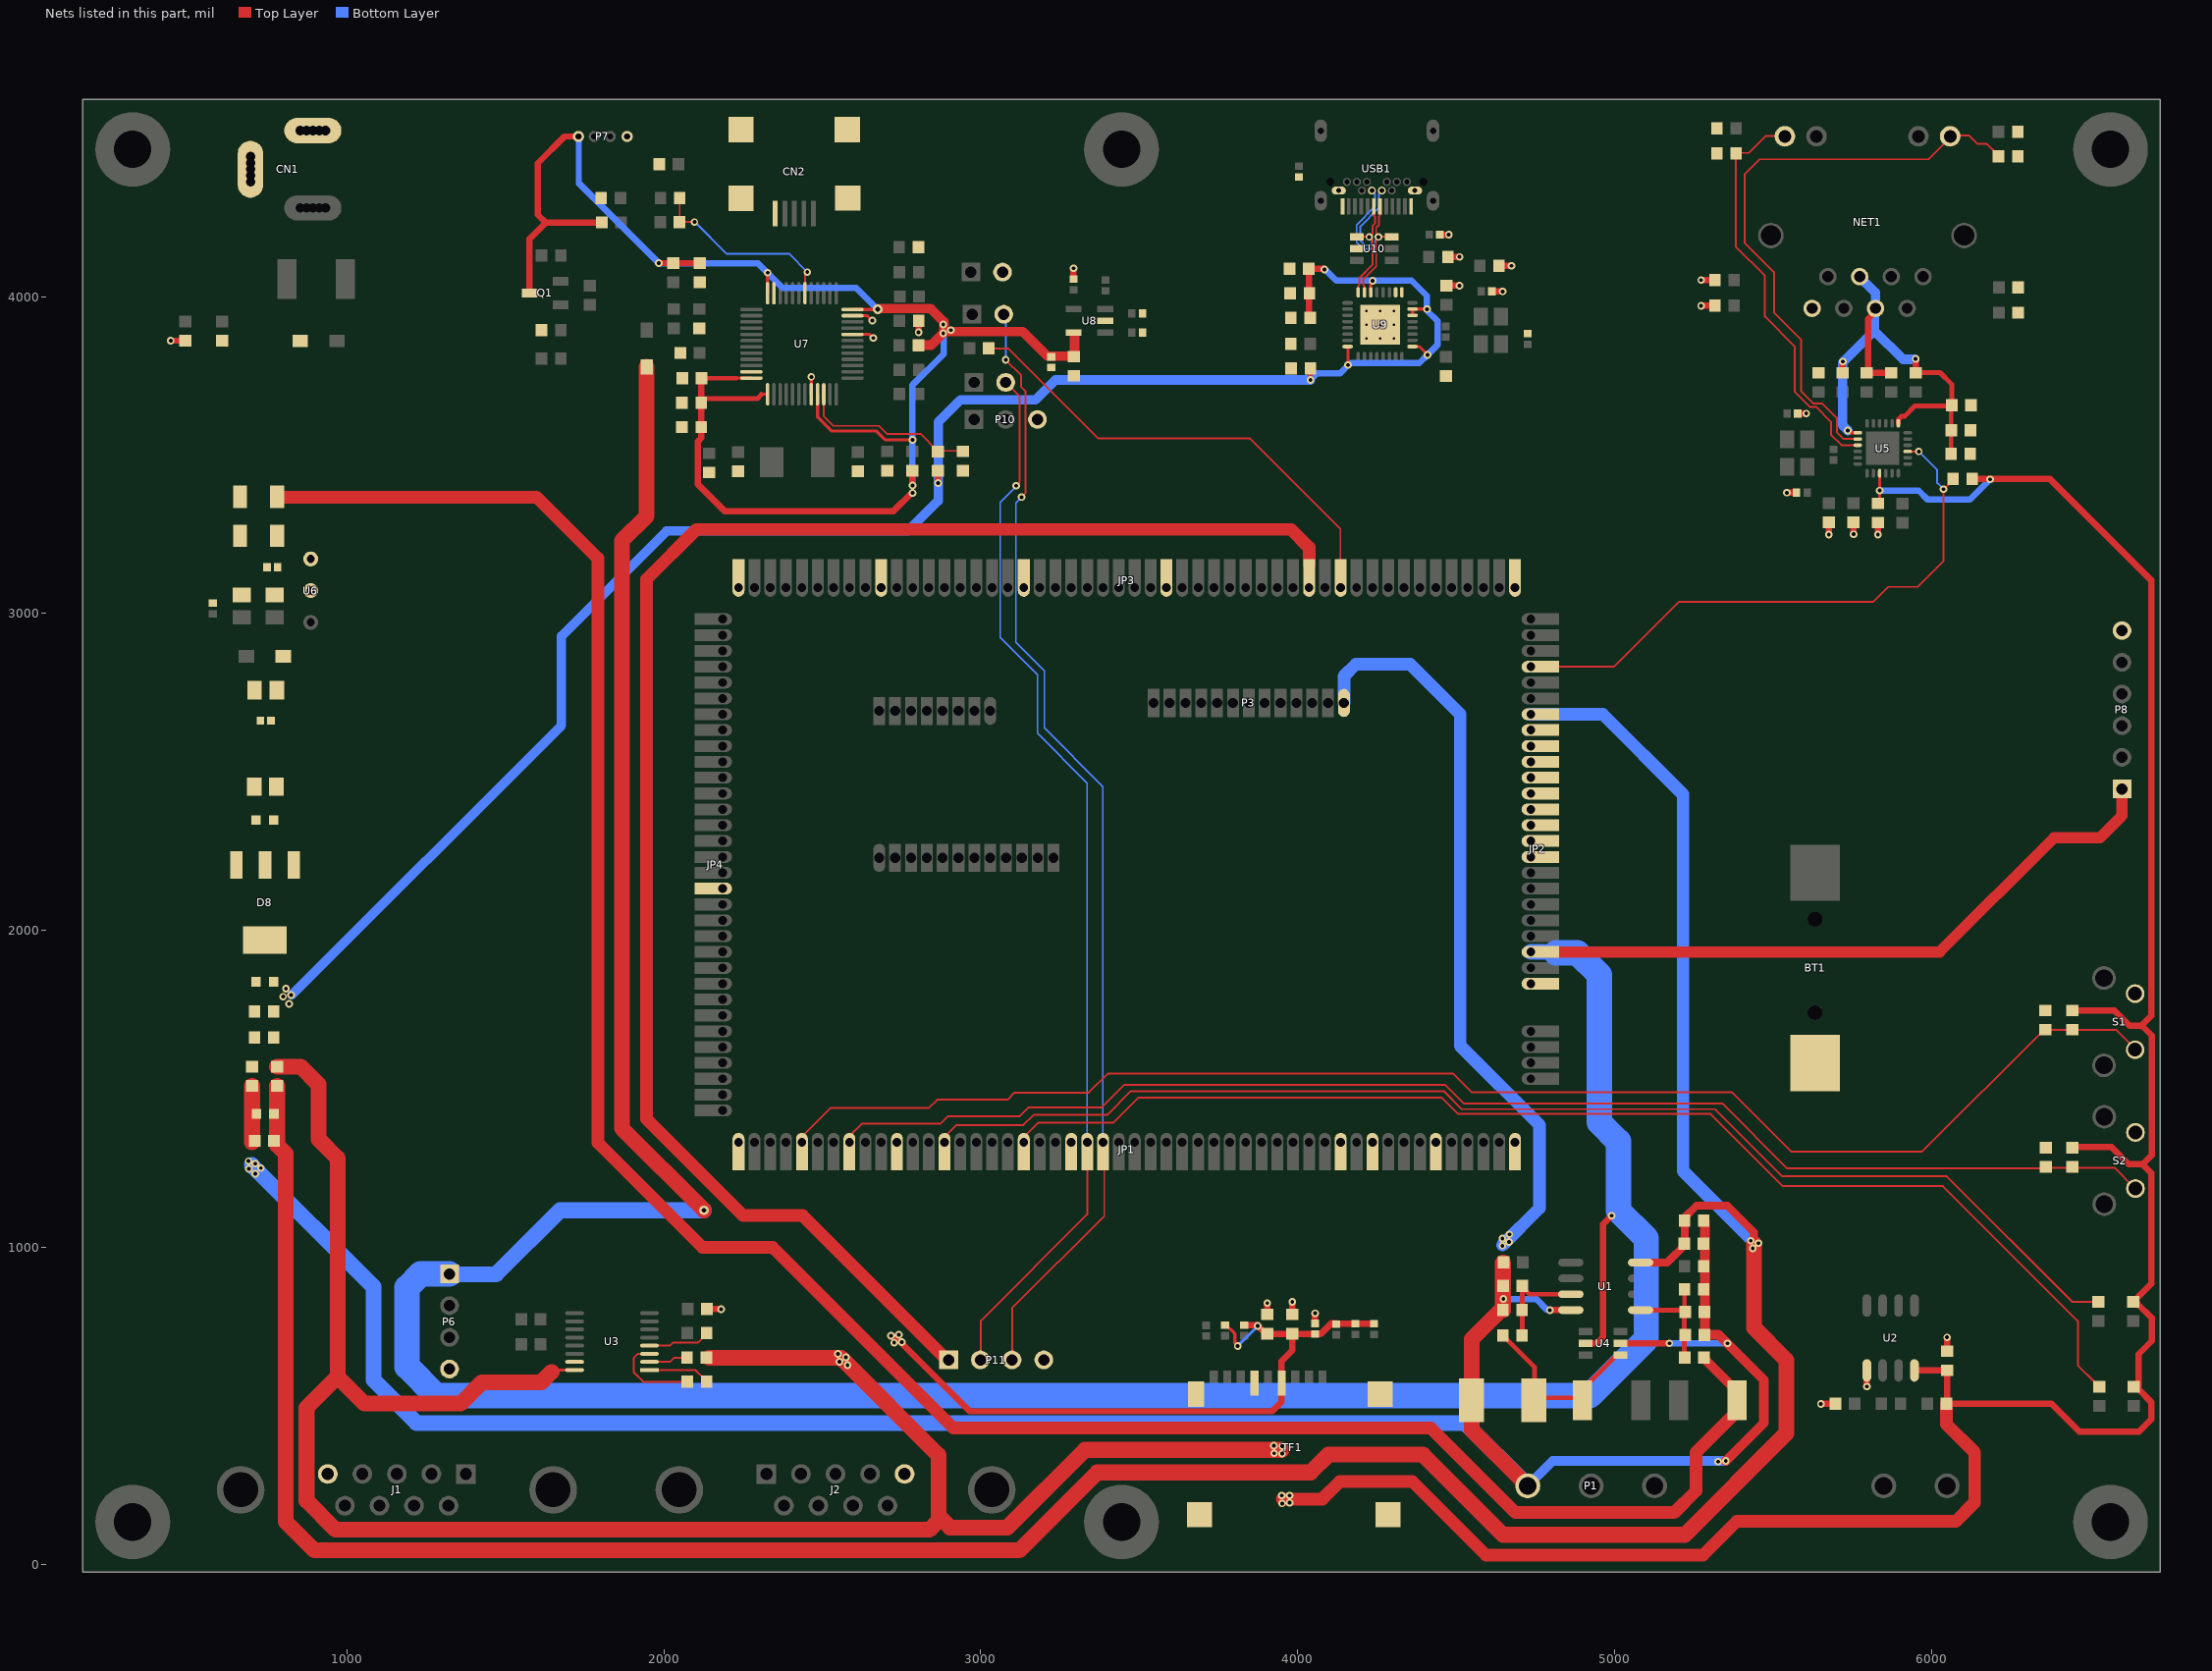
[diagram p0: the nets of this part, all layers, seen from the top]
# Altium PCB MISC105202-15.PcbDoc (part 2 of 4)
Units mil, origin at the board's own origin, x right, y up, seen from the top; angles counter-clockwise.
Board outline 6555.12 x 4645.67 mil, 2 copper layers (Top Layer, Bottom Layer); 182 components, 258 nets, 994 pads, 145 vias.
Unrouted connection lines stored in the file: 1.

## Footprints (in the part's own frame and the unit in brackets; to place one, negate y for a bottom-side part, rotate by r counter-clockwise, add the part's x,y. Pads: shape width x height; smd on the part's side, far side on the other; paste and mask are expansions set on the pad) (continued)
SMD-3225_4P [mm]
  rect 1.4x1.15 smd: 1(-1.1,-0.8) 2(1.1,-0.8) 3(1.1,0.8) 4(-1.1,0.8)
  silkscreen extent -2.1,-2.35 2.1,1.7, body extent -1.6,-1.25 1.6,1.25, height 0.61
SMD-5032_2P [mm]
  rect 1.9x2.4 smd: 1(-2.05,0) 2(2.05,0)
  silkscreen extent -3.32,-1.6 3.32,1.6
SO-8 [mil]
  oval 80x24 smd: 1(0,0) 2(0,-50) 3(0,-100) 4(0,-150) 5(220,-150) 6(220,-100) 7(220,-50) 8(220,0)
  silkscreen extent 60,-175 160,25
SOD-123 [mm]
  rect 1.25x1 smd: 1(1.475,0) 2(-1.475,0)
  silkscreen extent -0.5,-0.7 0.5,0.7, body extent -1.85,-0.77 1.85,0.78, height 1.35
SOIC-8_150mil [mm]
  oval 0.7x1.8 smd: 1(-1.905,-2.6) 2(-0.635,-2.6) 3(0.635,-2.6) 4(1.905,-2.6) 5(1.905,2.6) 6(0.635,2.6) 7(-0.635,2.6) 8(-1.905,2.6)
  silkscreen extent -2.9,-3.05 2.4,1.4
SOT23-5 [mil]
  rect 20x50 smd: 1(74.8,100) 2(37.4,100) 3(0,100) 4(0,0) 5(74.8,0)
  silkscreen extent 30,-5 45,-5
SOT-23(SOT-23-3) [mm]
  rect 1.25x0.7 smd: 1(1.25,-0.95) 2(1.25,0.95) 3(-1.25,0)
  silkscreen extent -0.65,-1.46 0.9,1.46, body extent -1.5,-1.5 1.5,1.5, height 1.3
SOT-23-6 [mm]
  rect 1.1x0.6 smd: 1(1.4,-0.95) 2(1.4,0) 3(1.4,0.95) 4(-1.4,0.95) 5(-1.4,0) 6(-1.4,-0.95)
  silkscreen extent -0.5,-1.87 1.73,1.4
SOT-223 [mm]
  rect 2.2x1 smd: 1(3,-2.3) 2(3,0) 3(3,2.3)
  rect 2.2x3.5 smd: 2(-3,0)
  silkscreen extent -1.4,-3 1.4,3, body extent -3.49,-3.24 3.49,3.24, height 1.64
TSSOP-16 [mm]
  rect 1.5x0.3 smd: 1(0,0)
  oval 1.5x0.3 smd: 2(0,-0.65) 3(0,-1.3) 4(0,-1.95) 5(0,-2.6) 6(0,-3.25) 7(0,-3.9) 8(0,-4.55) 9(6,-4.55) 10(6,-3.9) 11(6,-3.25) 12(6,-2.6) 13(6,-1.95) 14(6,-1.3) 15(6,-0.65) 16(6,0)
  silkscreen extent 1.58,-5.08 4.42,0.33
USB_TYPEC [mm]
  oval 1x1.8 hole 0.5 slot 1.3 at 90 deg: 0(-4.5,-2.805) 0(4.5,-2.805)
  oval 1x1.6 hole 0.5 slot 1.1 at 90 deg: 0(-4.5,2.805) 0(4.5,2.805)
  oval 0.64x0 hole 0.64 slot 0.95 at 0 deg unplated: 0(-3.725,1.295) 0(3.725,1.295)
  rect 0.3x1.3 smd: A1(-2.75,3.243) A2(-2.25,3.243) A3(-1.75,3.243) A4(-1.25,3.243) A5(-0.75,3.243) A6(-0.25,3.243) A7(0.25,3.243) A8(0.75,3.243) A9(1.25,3.243) A10(1.75,3.243) A11(2.25,3.243) A12(2.75,3.243)
  oval 1.14x0.64 hole 0.4 slot 0.9 at 0 deg: B1(3.05,1.995) B12(-3.05,1.995)
  round 0.65 hole 0.4: B2(2.4,1.295) B3(1.6,1.295) B4(1.2,1.995) B8(-0.8,1.295) B10(-1.6,1.295) B11(-2.4,1.295)
  round 0.64 hole 0.4: B5(0.8,1.295) B6(0.4,1.995) B7(-0.4,1.995) B9(-1.2,1.995)
  silkscreen extent -4.5,-6.46 4.5,3.96
ZY78xxLS-1000 [mm]
  round 1.2 hole 0.65: 1(-2.54,0) 2(0,0) 3(2.54,0)
  silkscreen extent -6,0.69 6,18.2

## Part data
BT1: library part Battery, "Multicell Battery"
C1 C2 C5 C6: library part "0603 100pF (101) 5% 50V", "贴片电容"
C3 C12 C25: library part "0603 10uF (106) 10% 10V", "贴片电容"
C4 C10 C22 C23 C24 C26 C58 C59 C60 C61 C62 C65 C66 C67: library part "0603 100nF (104) 10% 50V", "贴片电容"
C7 C8 C9 C11: library part CAP
C13 C14 C40 C41 C43: library part "0603 22uF (226) 20% 6.3V", "贴片电容"
C15 C30 C33 C35: library part "0402 100nF (104) 10% 16V", "贴片电容"
C16: library part "0603 22nF (223) 10% 50V", "贴片电容"
C17 C18 C20 C21: library part "0603 10pF (100) 5% 50V", "贴片电容"
C19 C28: library part "0402 10nF (103) 10% 50V", "贴片电容"
C27 C29 C54 C55 C57: library part "Cap Semi", "Capacitor (Semiconductor SIM Model)"
C31 C32 C34 C38: library part "0805 22uF (226) 20% 25V", "贴片电容"
C36 C37: library part "1206 10uF (106) 10% 50V", "贴片电容"
C39 C42 C44: library part CAP, "Capacitor"
C46 C47 C48 C49 C50 C51 C52: library part Capacitor_ST, "Capacitor 0402 / 0603 / 0805"
C53: library part "Cap Pol1", "Polarized Capacitor (Radial)"
C56: library part "0402 10uF (106) 20% 6.3V", "贴片电容"
C63 C64: library part "0402 20pF (200) 5% 50V", "贴片电容"
CN1: library part PJ202A
CN2: library part Mini-USB-AB
D3: library part "D Tunnel2", "Tunnel Diode - Dependent Source Model"
D4 D14: library part "0603 绿灯", "发光二极管"
D5 D9 D13: library part "0603 红灯", "发光二极管"
D6 D7 D12: library part "SOD-123 B5819W  SL", "肖特基二极管"
D8: library part CL1117-33
F1 F2 F3: library part "Fuse 2", "Fuse"
J1 J2: library part "D Connector 9", "Receptacle Assembly, 9 Position, Right Angle"
JP1 JP3: "Header, 50-Pin"
JP5 JP6: library part JP2
L1 L2: library part "0603 4.7uH 10%", "贴片电感"
P1 P10: library part "Header 3", "Header, 3-Pin"
P2 P9: library part "Header 2", "Header, 2-Pin"
P3: "Header, 13-Pin"
P4: "Header, 12-Pin"
P5: "Header, 8-Pin"
P6 P7 P11: library part "Header 4", "Header, 4-Pin"
P8: library part "Header 6", "Header, 6-Pin"
Q1: library part "SOT-23 SS8050 Y1", "三极管"
R1 R2 R3 R4 R28 R30 R31 R52: library part "0603 10KΩ (1002) 1%", "贴片电阻"
R5 R7: library part "0603 360Ω (3600) 1%", "贴片电阻"
R6: library part "0603 120Ω (1200) 1%", "贴片电阻"
R8 R9: library part "0603 100Ω (1000) 1%", "贴片电阻"
R11 R12 R13 R14 R15: library part "0402 47KΩ (4702) 1%", "贴片电阻"
R16: library part "0402 100Ω (1000) 1%", "贴片电阻"
R17 R19 R32 R57 R58 R59: library part Reszte, "Resistor"
R18 R20: library part "0603 680Ω (6800) 1%", "贴片电阻"
R21 R22 R23 R24: library part "0603 49.9Ω (49R9) 1%", "贴片电阻"
R25 R26 R29 R50 R51: library part "0603 510Ω (5100) 1%", "贴片电阻"
R27 R61: library part "0603 12KΩ (1202) 1%", "贴片电阻"
R33: library part RES-S
R34 R35 R48 R49 R54 R56: library part Res1, "Resistor"
R36 R37 R38 R39 R40 R41 R42 R43 R44 R45 R46 R47 R53 R55: library part Resistor_ST, "Resistor 0402 / 0603 / 0805"
R60: library part "0402 1MΩ (1004) 1%", "贴片电阻"
S1 S2: library part SW-PB
U1: library part OPA2335
U2: library part SP3485EN-L/TR_[C8963], "RS-485/RS-422"
U3: "RS232"
U4: library part SRV05-4-P-T7_[C85364], "TVS"
U5: library part LAN8742A-CZ-TR, "LAN8742A-CZ-TR - Small Footprint RMII 10/100 Ethernet, Transceiver with HP Auto-MDIX and flexPWR Technology SQFN-24"
U6: library part ZY78xxLS
U7: "Medium-density performance line ARM-based 32-bit MCU with 64KB Flash"
U8: library part TPS76901HDB
U9: library part USBD3300
U10: library part TPD4E001
USB1: library part USB_Type_C_Receptacle
Y1 Y3: library part "SMD-3225_4P  25MHZ 12PF 10PPM", "贴片晶振"
Y2: library part "SMD-5032_2P 8MHz 20ppm 20pF", "贴片晶振"

## Free pads (board coordinates)
  round 236.22 hole 118.11: 0(324.48,133.48) 0(324.48,4464.19) 0(3444.56,133.48) 0(3444.56,4464.19) 0(6564.64,133.48) 0(6564.64,4464.19)

## Via types
v1: diameter 24, hole 12, Top Layer to Bottom Layer, 128 vias
v2: diameter 19.68, hole 7.87, Top Layer to Bottom Layer, 9 vias
v3: diameter 50, hole 50, Top Layer to Bottom Layer, 4 vias
v4: diameter 30, hole 15, Top Layer to Bottom Layer, 2 vias
v5: diameter 137.8, hole 137.8, Top Layer to Bottom Layer, 2 vias

## Nets (pads, with @x,y where several pads share a name; then routed paths per layer and width w, separated by ;. In a path a pad name is that pad's centre, name@x,y a point inside that pad or via, vN(x,y) a via of type N, cw(c..) or ccw(c..) an arc to the next point about the centre after c; other vN are vias at no path point)
3V3: C8.1 C10.2 C13.2 C14.2 C15.2 C22.2 C40.2 C41.2 C42.2 C59.2 C60.2 C61.2 C62.2 D4.A D5.A D8.2 L1.1 R5.1 R11.2 R12.2 R13.2 R14.2 R15.2 R17.2 R19.2 R28.1 R43.1 TF1.4 U2.8 U3.16 U5.9 U9.6 U9.16 U9.25 U9.30 U9.31 | length 22661.3
  Top Layer w10: 1636,601 1648,613 U3.16@1718.78,613 ; R13.2@3771,754.73 3774.87,754.73 3802,727.6 3802,698 v1(3811,689) ; U9.16@4157.64,3842.1 4159,3840.74 v1(4159,3784) ; U9.6@4230.47,4013.36 4230.47,4043.47 v1(4237,4050) ; U9.25@4362.36,3842.1 4383.9,3842.1 v1(4410,3816) ; U9.30@4363,3943 4362.36,3943.64 U9.31@4362.36,3960.21 v1(4408.21,3960.21) ; C22.2@5836.16,3359.16 v1@5836.16,3393 ; v1(5836.16,3387.84) v1@5836.16,3393 ; U5.9@5836.16,3442.26 v1@5836.16,3393
  Top Layer w15: v1(4040.31,3736.69) C62.2@4040.31,3773
  Top Layer w20: C8.1@2134.31,652 C8.1@2144,652 ; v1@2716.5,718.5 2729.5,718.5 2965.44,482.56 3919.56,482.56 3949.69,512.69 TF1.4@3949.69,571.56 3949.69,641.69 3983,675 C13.2@3983,716 ; v1(2865.43,3411.57) R43.1@2865.43,3450.31 ; 2871,142 2874,145 ; R12.2@3831,754.73 3872.27,754.73 C14.2@3896,731 ; C14.2@3904,727.68 3904.69,727 4054,727 C15.2@4055,726 ; C61.2@4035,3931 4035.31,3931.31 C59.2@4035.31,4088 4082,4088 v1@4083,4087 ; C15.2@4059,726 4072,726 4106,760 4122,760 4123.27,758.73 R14.2@4182,758.73 R11.2@4241,758.73 ; U2.8@5946,611.64 6047.36,611.64 6049,610 6049,519 R5.1@6053,515 ; R5.1@6047.31,506 6379,506 6466,419 6655,419 6693,457 6693,512 6653,552 6653,663 6695,705 6695,777 D4.A@6649,823 ; R28.1@6128.31,3424 6374,3424 6693,3105 6693,1730 6662,1699 ; R17.2@6454,1747 6577,1747 6625,1699 6662,1699 ; R19.2@6455,1316 6568,1316 6622,1262 6666,1262 ; D4.A@6636,827.87 6693,884.87 6693,1235 6666,1262 ; D4.A@6644,826 D4.A@6649,826 ; 6661,1698 6662,1699 ; 6662,1699 6664,1699 6695,1668 6695,1291 6666,1262
  Top Layer w40: v1@3951,206 4078,206 4133,261 4362,261 4594,29 5279,29 5386,136 6077,136 6136,195 6136,353 6047.31,441.69 R5.1@6047.31,506
  Top Layer w50: L1.1@780,1570.31 854.69,1570.31 911,1514 911,1341 971,1281 971,592 ; 1646,607 1613,574 1426,574 1359,507 1056,507 971,592 ; C8.1@2144,652 2559,652 2867,344 2867,138 2838,109 965,109 873,201 873,494 971,592 ; 2874,145 2903,116 3084,116 3329,361 3949,361
  Bottom Layer w10: v1(3811,689) v1(3874,752)
  Bottom Layer w20: v1@4040,3736 4061,3757 4133,3757 4166,3790 4384,3790 v1(4410,3816) 4441,3847 4441,3923 4408,3956 4408,4002 4360,4050 v1(4237,4050) 4122,4050 v1@4087,4085 ; v1(4085,4085) v1@4086,4084 ; v1(5836.16,3387.84) 5959.16,3387.84 5988,3359 6121,3359 v1(6185,3423)
  Bottom Layer w30: v1@826.5,1796.5 1677,2647 1677,2928 2009,3260 2770,3260 2866,3356 2866,3604 2936,3674 3173,3674 3235.69,3736.69 v1(4040.31,3736.69)
  other v1: 3951,192 3975,194 3950,217 3975,217 3951,349 3926,350 3952,373 3925,374 2580,628 2554,639 2575,653 2550,664 2727,699 2751,701 2717,721 2742,724 818,1768 799,1791 824,1796 808,1816
3V3_E: C16.1 C23.2 C24.2 NET1.4 NET1.5 R21.2 R22.2 R23.2 R24.2 U5.1 U5.19 | length 1630.2
  Top Layer w10: v1(5736,3577) 5742.79,3570.21 U5.1@5767.26,3570.21
  Top Layer w15: U5.19@5895.21,3599.74 5895.21,3612.21 5905,3622 5915,3622 5948,3655 C16.1@6061,3655 ; R23.2@5962,3760 6027,3760 6063.68,3723.31 C16.1@6063.68,3657 ; C23.2@6061.68,3503 C16.1@6061.68,3650.69
  Top Layer w20: R22.2@5720,3759.32 v1(5720,3795) ; NET1.4@5825,3955 5799.68,3929.68 5799.68,3759.32 R24.2@5873,3759.32 ; R23.2@5950,3759.32 v1(5950,3803)
  Bottom Layer w30: v1(5736,3577) 5719,3594 5719,3791 5820,3892 ; NET1.5@5773.2,4062.63 5823,4012.83 NET1.4@5823,3971 ; NET1.4@5820,3962 5820,3892 ; v1@5947,3802 5910,3802 5820,3892
+3V3: JP3.37 P11.1 | length 5210.4
  Top Layer w30: JP3.37@4036,3147 JP3.37@4036,3155
  Top Layer w40: P11.1@2899,645 2893,645 2438,1100 2251,1100 1946,1405 1946,3108 2103,3265 3979,3265 4036,3208 JP3.37@4036,3155
+3V3_ST_LINK: C46.2 C47.2 C48.2 C49.2 C55.2 C56.2 D14.A P7.1 Q1.3 R38.1 R41.2 R49.1 U7.1 U7.9 U7.24 U7.36 U7.48 U8.5 | length 5585.1
  Top Layer w10: 2230,3742.73 U7.48@2276.55,3742.73 ; 2307.45,3691.55 U7.1@2327.73,3691.55 ; U7.36@2327.73,4010.45 v1(2327.73,4075.27) ; U7.9@2485.21,3691.55 2485.21,3619.79 2529,3576 2670,3576 2698,3548 v1(2785,3548) ; U7.24@2595.45,3959.27 2645.73,3959.27 2646,3959
  Top Layer w12: 2646,3959 v4@2677,3959
  Top Layer w15: C48.2@2119.31,3733.31 C48.2@2119.31,3742 2230,3742 ; C49.2@2132,3678 2296,3678 2307.45,3689.45 2307.45,3691.55
  Top Layer w20: Q1.3@1576.79,4011 1576.79,4181.79 1628,4233 ; P7.1@1728,4505 1687,4505 1603,4421 1603,4258 1628,4233 ; D14.A@1804,4235 1802,4233 1628,4233 ; v1(1984.31,4105.31) R38.1@2030,4105.31 ; R38.1@2035,4108 2037.69,4105.31 C46.2@2114,4105.31 ; C48.2@2122,3736 2119.31,3733.31 2118,3732 2118,3656 2118.31,3655.69 C47.2@2118.31,3588 2118.31,3553.31 2108,3543 2108,3407 2192,3323 2725,3323 v1@2783.5,3381.5 ; v1(2785,3404) R41.2@2785,3450.68
  Top Layer w30: v4@2677,3961 2677.71,3961.71 2842.29,3961.71 2884,3920 2884,3887 2844,3847 R49.1@2810,3847 ; v1@2886,3889 3133,3889 3210,3812 3291,3812 3296,3817 U8.5@3296,3880
  Bottom Layer w20: P7.1@1732,4502 1732,4357.63 v1(1984.31,4105.31) 1983,4104 2298,4104 2311,4091 ; v1@2325,4077 2311,4091 ; v4(2675,3960) 2674,3960 2607,4027 2375,4027 2311,4091 ; v1(2785,3404) v1(2785,3548) 2785,3721 2884,3820 v1@2884,3882
  other v1: 2785,3380 2882,3884 2906,3894 2882,3912
+5V: C34.2 C35.1 C38.2 C39.2 D7.2 D8.1 D12.1 JP2.11 P6.1 P8.1 U4.5 | length 12105.7
  Top Layer w20: U4.5@4907.88,697 4944,697 4964,717 4964,1073 v1(4991,1100)
  Top Layer w35: JP2.11@4780.49,1931.87 6025.87,1931.87 6386,2292 6531,2292 6601,2362 P8.1@6601,2436
  Top Layer w50: D12.1@1946,3777.93 1946,3307 1868,3229 1868,1376 v4(2127,1117)
  Bottom Layer w50: P6.1@1317,915 1471,915 1673,1117 v4(2127,1117) ; JP2.11@4736,1931.87 4811.87,1931.87 4816,1936
  Bottom Layer w80: P6.1@1324,916 1233,916 1190,873 1190,624 1282,532 4922,532 5100,710 5100,760 5100,1028 5012,1116 5012,1334 4952,1394 4952,1860 4883,1929 4816,1929
A3V3: C3.2 C4.2 C43.2 C44.2 JP2.26 L1.2 U1.8 | length 9790.7
  Top Layer w25: U1.8@5082,952 5166,952 5221,1007 5221,1094 5258,1131 5356,1131 5439,1048 v1@5439,1027
  Top Layer w50: L1.2@780,1509.68 780,1323 807,1296 807,135 898,44 3122,44 3368,290 4041,290 4097,346 4395,346 4648,93 5222,93 5542,413 5542,644 5440,746 5440,1012
  Bottom Layer w40: JP2.26@4736,2681.87 4963.13,2681.87 5216,2429 5216,1241 5441,1016
  other v1: 5436,997 5454,1013 5430,1021
AGND: C1.1 C2.1 C3.1 C4.1 C5.1 C6.1 C12.1 C43.1 C44.1 D3.1 L2.2 P1.3 P3.1 R2.1 R4.1 U1.4 U4.2 | length 10084.7
  Top Layer w20: v1(4796,802) U1.4@4862,802 ; U4.2@5018.12,697 v1(5173,697)
  Top Layer w30: C4.1@5282,1086 5285,1083 5285,940 5285,725.68 C12.1@5283.31,724 5328,724 5471,581 5471,446 v1(5351,326)
  Top Layer w50: C43.1@701,1331 701,1336 L2.2@701,1509.68 ; R2.1@4643,804 4549,710 D3.1@4549,518 4549,424 P1.3@4717,256 ; R2.1@4647.69,802 4647.69,950.69 C1.1@4648,951
  Bottom Layer w20: v1(4649,837) 4753,837 4788,802 v1(4796,802) ; v1(5173,697) v1(5356,697)
  Bottom Layer w30: P1.3@4737,258 4805,326 v1(5351,326)
  Bottom Layer w40: P3.1@4146,2717.62 4146,2802 4184,2840 4355,2840 4513,2682 4513,1636 4763,1386 4763,1124 v1@4646,1007
  Bottom Layer w50: v1@700,1260 1084,876 1084,582 1220,446 4527.37,446 P1.3@4726,247.37
  other v1: 5327,324 4646,1005 4667,1017 4646,1028 4668,1041 711,1232 691,1248 729,1250 711,1264 690,1272
AIN1: D3.2 F1.2 R1.2 U4.1 | length 560.6
  Top Layer w15: R1.2@4647.68,722 4748,621.68 D3.2@4748,559 ; D3.2@4761,523 4763,525 F1.2@4898,525 ; F1.2@4898,518 F1.2@4898,525 ; F1.2@4918,543 4900,525 F1.2@4898,525 ; U4.1@5011,659 5006,659 4898,551 F1.2@4898,525
AIN2: C30.1 C36.2 C37.2 D6.2 F3.2 R3.2 R33.1 U6.1 | length 7419.2
  Top Layer w30: R3.2@5287,645 5387,545 F3.2@5387,518 F3.2@5387,483
  Top Layer w40: C36.2@782,3367 1599,3367 1792,3174 1792,1330 2122,1000 2344,1000 2914,430 4420,430 4687,163 5188,163 5257,232 5257,353 F3.2@5387,483
AIN_1: R43.2 R44.2 U7.10 | length 549.7
  Top Layer w6: U7.10@2504.9,3691.55 2504.9,3622.1 2535,3592 2679,3592 2704,3567 2810,3567 2864,3513 R44.2@2940,3513
ARM_NRST: JP3.39 R36.2 | length 1477.4
  Top Layer w6: R36.2@3025.32,3836 3087,3836 3371,3552 3440,3552 3850,3552 4135,3267 JP3.39@4135,3135
ARM_SWO: R37.2
ARM_TCK: JP1.23 JP5.2 P11.2 | length 3318.1
  Top Layer w6: P11.2@3001,661 3001,769 3336,1104 JP1.23@3336,1287.38 ; JP5.2@3079,3729 3123,3685 3123,3414 v1(3112,3403)
  Bottom Layer w4: 3061.3,3230.7 3061.3,3229 ; v1@3111,3400 3061.3,3350.3 3061.3,3229 ; JP1.23@3336,1331.87 3336,2465 3179,2622 3179,2807 3061.3,2924.7 3061.3,3229
ARM_TMS: JP1.24 JP6.2 P11.3 | length 3539.5
  Top Layer w6: v1(3079,3800) 3128,3751 3128,3715 3142,3701 3142,3380 v1(3129,3367) ; P11.3@3099,645 3099,808 3390,1099 JP1.24@3390,1317
  Bottom Layer w4: v1(3129,3367) 3111,3349 3111,2909 3201,2819 3201,2639 3386,2454 3386,1380 JP1.24@3386,1331.87
  Bottom Layer w6: v1(3079,3800) JP6.2@3079,3926
BOOT0: JP1.41
D_N: U9.8 U10.1 USB1.A7 USB1.B7 | length 598.1
  Top Layer w6: U10.1@4186.88,4188.4 4225.6,4188.4 4236,4198.8 4236,4222 4244,4230 4244,4252.16 4240.16,4256 USB1.A7@4240.16,4284.95 ; U9.8@4191.1,4013.36 4191.1,4034 4194.94,4037.84 4194.94,4058.92 4236,4099.97 4236,4178 v1(4226,4188)
  Bottom Layer w6: v1@4225,4188 4235,4178 4235,4166.97 4230.03,4162 4211.97,4162 4198,4175.97 4198,4221.03 4256,4279.03 4256,4324.34 USB1.B7@4265.75,4334.09
D_P: U9.7 U10.6 USB1.A6 USB1.B6 | length 603.1
  Top Layer w6: U9.7@4210.79,4013.36 4210.79,4034 4206.94,4037.84 4206.94,4053.94 4248,4095 4248,4177 ; 4248,4199 4248,4217.03 4256,4225.03 4256,4252.16 4259.84,4256 USB1.A6@4259.84,4284.95 ; v1@4259.4,4188.4 U10.6@4297.12,4188.4
  Bottom Layer w6: USB1.B6@4234.25,4334.09 4244,4324.34 4244,4284 4186,4226 4186,4171 4207,4150 4235,4150 4246,4161 4246,4179 v1@4253,4186
  other v1: 4255,4188
DSI_CK_N: JP2.23
DSI_CK_P: JP2.24
DSI_D0_N: JP2.20
DSI_D0_P: JP2.21
DSI_D1_N: JP2.17
DSI_D1_P: JP2.18
ETH_RESET: JP2.29 R28.2 U5.15 | length 1838.7
  Top Layer w6: JP2.29@4780.49,2831.87 4997.87,2831.87 5203,3037 5817,3037 5864,3084 5956,3084 6038,3166 6038,3391 R28.2@6060,3413 ; U5.15@5924.74,3511.16 v1(5959.84,3511.16)
  Bottom Layer w6: v1(5959.84,3511.16) 6018,3453 6018,3412 v1(6038,3392)
GND: BT1.2 C10.1 C11.1 C13.1 C14.1 C15.1 C16.2 C17.2 C18.2 C19.2 C20.2 C21.2 C22.1 C23.1 C24.1 C25.1 C26.1 C27.2 C28.2 C29.2 C30.2 C31.1 C32.1 C33.2 C34.1 C35.2 C36.1 C37.1 C38.1 C39.1 C40.1 C41.1 C42.1 C46.1 C47.1 C48.1 C49.1 C50.2 C51.2 C52.1 C53.2 C54.1 C55.1 C56.1 C57.1 C58.1 C59.1 C60.1 C61.1 C62.1 C63.2 C64.2 C65.1 C66.1 C67.1 CN1.2 CN1.3 CN2.0 CN2.5 D8.3 D9.K D13.K J1.5 J2.5 JP1.1 JP1.11 JP1.22 JP1.39 JP1.45 JP1.50 JP2.9 JP2.19 JP2.22 JP2.25 JP3.1 JP3.10 JP3.19 JP3.28 JP3.50 JP4.15 L2.1 NET1.8 P6.4 P7.4 P8.6 P9.2 P10.3 P11.4 R7.1 R25.2 R26.2 R27.2 R30.2 R31.1 R35.2 R39.1 R40.1 R44.1 R48.2 R52.1 R56.1 R58.2 R59.1 R61.1 S1.2 S2.2 TF1.0 TF1.6 U2.5 U3.15 U6.2 U7.8 U7.20 U7.23 U7.35 U7.47 U8.2 U9.1 U9.2 U9.33 U10.2 USB1.A1 USB1.A12 USB1.B1 USB1.B12 | length 1040.8
  Top Layer w10: U7.8@2465.53,3691.55 v1(2465.53,3746.47) ; U7.20@2595.45,3880.53 2649.47,3880.53 v1(2661,3869) ; U7.23@2595.45,3939.58 2642.42,3939.58 v1(2658,3924)
  Top Layer w20: v1(444.31,3860.69) D9.K@490,3860.69 ; C11.1@2136.31,805 v1(2181,805) ; v1(2804.32,3887.32) R48.2@2804.32,3923 ; C57.1@3293,4054.73 v1(3293,4089) ; C14.1@3904,788.32 v1(3904,824) ; C13.1@3983,788.32 v1(3983,828) ; C15.1@4055,759.73 v1(4055,792) ; R59.1@4448.73,4195 v1(4477,4195) ; C65.1@4470,4034.31 v1(4510.69,4034.31) ; C58.1@4474.31,4125 v1(4511,4125) ; C64.2@4612.73,4016 v1(4647,4016) ; R61.1@4635.31,4097 v1(4675,4097) ; v1(5273,3971) C21.2@5316.69,3971 ; v1(5273,4052) C20.2@5316.69,4052 ; v1(5544,3381) C29.2@5574.27,3381 ; C27.2@5577.73,3631 v1(5605,3631) ; v1(5651,506) R7.1@5696.69,506 ; v1(5676,3249) C25.1@5676,3287.69 ; v1(5754,3250) C26.1@5754,3287.69 ; v1(5796,561) U2.5@5796,611.64 ; v1(5831,3249) C22.1@5831,3286.69 ; C10.1@6049,672.32 v1(6049,716)
  other v2: 4216.69,3867.69 4260,3867.69 4303.31,3867.69 4216.69,3911 4260,3911 4303.31,3911 4216.69,3954.31 4260,3954.31 4303.31,3954.31
KEY1: C19.1 JP1.5 R17.1 S1.1 | length 4579.6
  Top Layer w6: JP1.5@2436,1331.87 2436,1344 JP1.5@2440.5,1348.5 ; JP1.5@2438,1351 2527,1440 2837,1440 2863,1466 3085,1466 3107,1488 3341,1488 3401,1548 4491,1548 4549,1490 5369,1490 5557,1302 5970,1302 6354,1686 6583,1686 S1.1@6635,1634
KEY2: C28.1 JP1.8 R19.1 S2.1 | length 4265.9
  Top Layer w6: JP1.8@2585,1350 2625,1390 2873,1390 2897,1414 3123,1414 3150,1441 3381,1441 3452,1512 4466,1512 4524,1454 5340,1454 5545,1249 6352,1249 6354,1251 6577,1251 S2.1@6637,1191 ; JP1.8@2586,1331.87 JP1.8@2586,1344
LED0: JP1.14 R18.2 | length 3989.8
  Top Layer w6: JP1.14@2886,1331.87 2886,1345 JP1.14@2888.5,1347.5 ; JP1.14@2887,1349 2924,1386 3135,1386 3167,1418 3399,1418 3474,1493 4461,1493 4518,1436 5317,1436 5528,1225 6047,1225 6444,828 R18.2@6525,828
LED1: JP1.19 R20.2 | length 3904
  Top Layer w6: JP1.19@3133,1345 3181,1393 3418,1393 3498,1473 4454,1473 4506,1421 5303,1421 5531,1193 6036,1193 6462,767 6462,628 R20.2@6516,574 ; JP1.19@3136,1331.87 JP1.19@3136,1346
LED_STLINK: R50.1 R51.1 U7.30 | length 617.8
  Top Layer w6: R51.1@2049.31,4235 v1(2097,4235) ; R50.1@2050.31,4310 2050.31,4233.69 R51.1@2054,4230 ; U7.30@2445.84,4010.45 2445.84,4069.84 v1(2453,4077)
  Bottom Layer w6: v1@2099,4234 2198,4135 2395,4135 v1(2453,4077)
LEDG-SPEED: NET1.9 R30.1 U5.2 | length 1877.5
  Top Layer w6: 5589,3837 5589,3834 ; U5.2@5767.26,3550.53 5722.47,3550.53 5701,3572 5701,3617 5655,3663 5627,3663 5589,3701 5589,3834 ; NET1.9@6055,4498 5990,4433 5458,4433 5410,4385 5410,4170 5503,4077 5503,3949 5589,3863 5589,3834 ; NET1.9@6071,4508 6119,4508 6145.5,4481.5 6174.5,4481.5 R30.1@6205,4451
LEDY-LINK: NET1.12 R31.2 U5.3 | length 1293.3
  Top Layer w6: NET1.12@5530,4506 5477,4506 5424,4453 5382,4453 5382,4158 5474,4066 5474,3937 5569,3842 5569,3699 5617,3651 5637,3651 5683,3605 5683,3564 5716.16,3530.84 U5.3@5767.26,3530.84
NetC2_2: C2.2 R1.1 R2.2 U1.3 | length 325.1
  Top Layer w15: C2.2@4705,885 4708.31,881.69 R1.1@4708.31,722 ; R1.1@4710,727 R1.1@4714,731 ; C2.2@4714,869 4731,852 U1.3@4862,852
NetC6_2: C6.2 C12.2 R3.1 R4.2 U1.5 | length 361.1
  Top Layer w15: U1.5@5082,802 R4.2@5220,802 ; C6.2@5220.69,868 5220.69,801.68 5220,801 5220,648 R3.1@5222,646
NetC7_1: C7.1 U3.1 | length 183.6
  Top Layer w6: U3.1@1955,613 2099,613 C7.1@2127,585
NetC7_2: C7.2 U3.3 | length 281.7
  Top Layer w6: U3.3@1955,664.18 1918.18,664.18 1906,652 1906,605 1935,576 C7.2@2074.69,576
NetC8_2: C8.2 U3.2 | length 116.1
  Top Layer w6: U3.2@1955,638.59 2019.59,638.59 2032,651 C8.2@2066,651
NetC9_1: C9.1 U3.4 | length 189.3
  Top Layer w6: U3.4@1955,689.77 2019.77,689.77 2029,699 2108,699 C9.1@2131,722